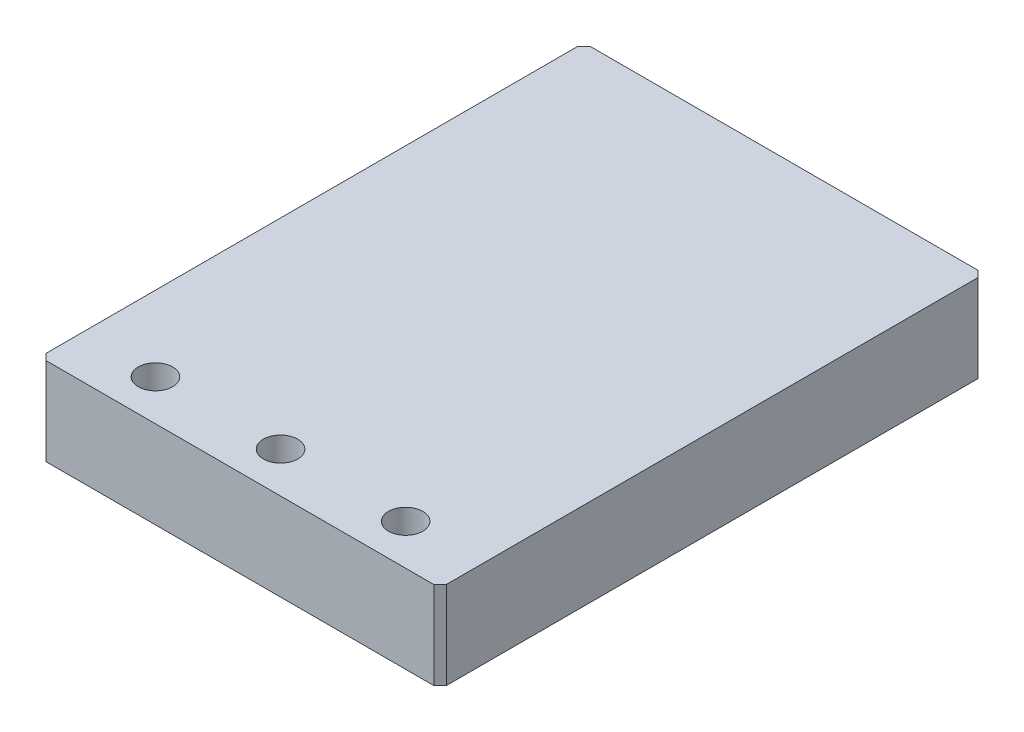
from build123d import *

# Parameters (mm, degrees)
SKETCH_1_W                  = 64
SKETCH_1_H                  = 14
EXTRUDE_1_DEPTH             = 87
HOLE_WIZARD_C_0_D           = 5.5
HOLE_WIZARD_C_0_CBORE_D     = 10
HOLE_WIZARD_C_0_CBORE_DEPTH = 5.5
HOLE_WIZARD_M6_1_D          = 5
HOLE_WIZARD_M6_1_DEPTH      = 13.5
HOLE_WIZARD_M6_1_TIP        = 1.502151548
CHAMFER_1_SIZE              = 1


with BuildPart() as part:
    # 草图1 → 凸台-拉伸1 (new body)
    with BuildSketch(Plane.XY):
        with Locations((10, -67.679969714)):
            Rectangle(SKETCH_1_W, SKETCH_1_H)
    extrude(amount=EXTRUDE_1_DEPTH)

    # 打孔尺寸根据六角头螺栓 C 级的类型0 (through all)
    with Locations(Plane(origin=(0, -74.679969714, 0), x_dir=(-1, 0, 0), z_dir=(0, -1, 0))):
        with Locations((10, -80.5), (-10, -80.5), (-30, -80.5)):
            CounterBoreHole(HOLE_WIZARD_C_0_D / 2, HOLE_WIZARD_C_0_CBORE_D / 2, HOLE_WIZARD_C_0_CBORE_DEPTH)

    # M6 螺纹孔1
    with Locations(Plane(origin=(0, 0, 0), x_dir=(-1, 0, 0), z_dir=(0, 0, -1))):
        with Locations((-30, -67.679969714), (-10, -67.679969714), (10, -67.679969714)):
            Hole(HOLE_WIZARD_M6_1_D / 2, depth=HOLE_WIZARD_M6_1_DEPTH)
            with Locations((0, 0, -(HOLE_WIZARD_M6_1_DEPTH + HOLE_WIZARD_M6_1_TIP / 2))):  # 118° drill point
                Cone(0, HOLE_WIZARD_M6_1_D / 2, HOLE_WIZARD_M6_1_TIP, mode=Mode.SUBTRACT)

    # 倒角1
    chamfer_1_edges = [part.edges().sort_by_distance(p)[0] for p in [
        (42, -67.679969714, 87),
        (-22, -67.679969714, 87),
        (42, -67.679969714, 0),
        (-22, -67.679969714, 0),
    ]]
    chamfer(chamfer_1_edges, length=CHAMFER_1_SIZE)


solid = part.part
